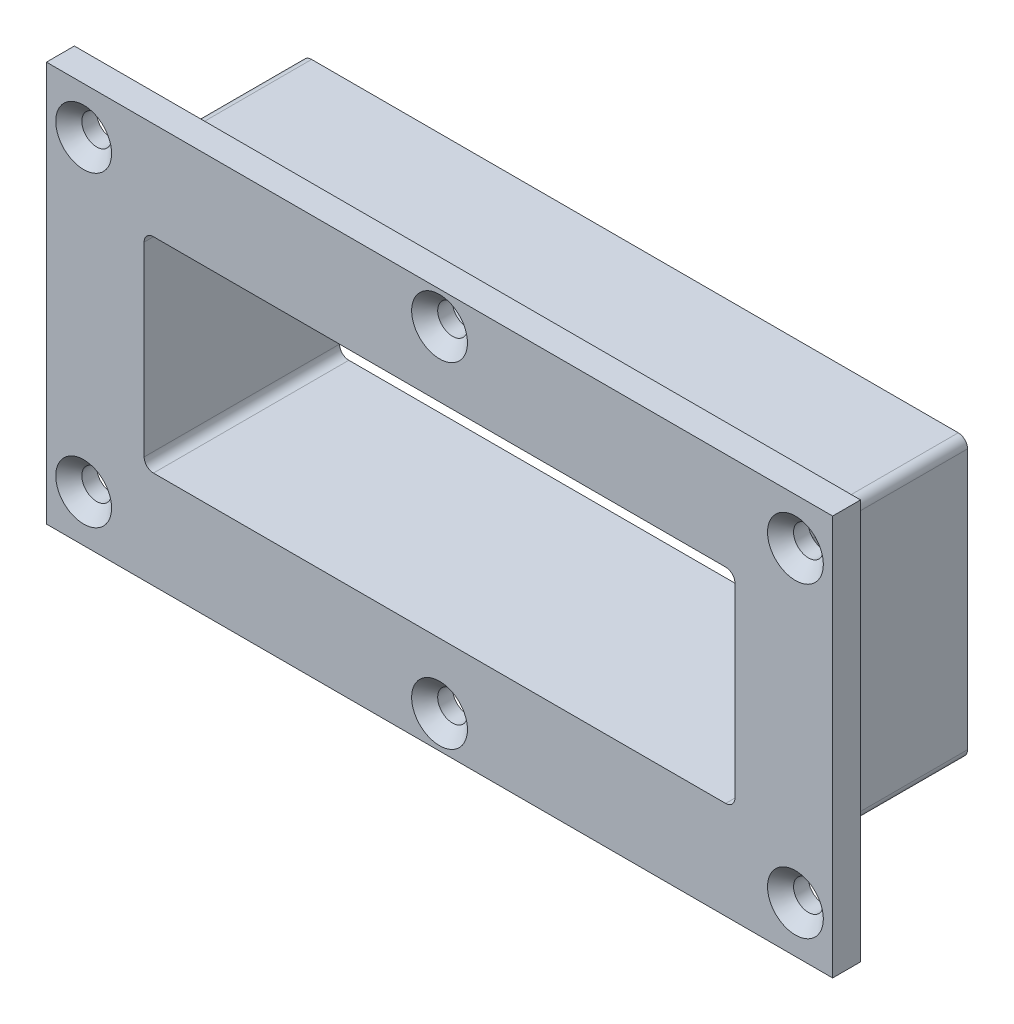
from build123d import *

# Parameters (mm, degrees)
SKETCH1_W                                         = 71.5
SKETCH1_H                                         = 30
SKETCH1_W_2                                       = 63.5
SKETCH1_H_2                                       = 22
BOSS_EXTRUDE1_DEPTH                               = 21
SKETCH2_W                                         = 71.5
SKETCH2_H                                         = 30
BOSS_EXTRUDE2_DEPTH                               = 3
SKETCH3_W                                         = 68.9
SKETCH3_H                                         = 27.4
SKETCH3_W_2                                       = 65.9
SKETCH3_H_2                                       = 24.4
CUT_EXTRUDE1_DEPTH                                = 1.5
SKETCH4_R                                         = 1.6
CUT_EXTRUDE2_DEPTH                                = 3
PILOT_HOLE_SIZE_PER_CROSS_FOR_HALF_CO_D           = 3.2
PILOT_HOLE_SIZE_PER_CROSS_FOR_HALF_CO_DEPTH       = 6.1
PILOT_HOLE_SIZE_PER_CROSS_FOR_HALF_CO_CSINK_D     = 6
PILOT_HOLE_SIZE_PER_CROSS_FOR_HALF_CO_CSINK_ANGLE = 90
PILOT_HOLE_SIZE_PER_CROSS_FOR_HALF_CO_TIP         = 0.96137699
FILLET1_R                                         = 1
FILLET2_R                                         = 1


with BuildPart() as part:
    # Sketch1 → Boss-Extrude1 (new body)
    with BuildSketch(Plane.XY):
        Rectangle(SKETCH1_W, SKETCH1_H)
        Rectangle(SKETCH1_W_2, SKETCH1_H_2, mode=Mode.SUBTRACT)
    extrude(amount=BOSS_EXTRUDE1_DEPTH)

    # Sketch2 → Boss-Extrude2 (add)
    with BuildSketch(Plane.XY.offset(21)):
        Polygon((42.25, 15), (42.25, -15), (42.25, -21.5), (-42.25, -21.5), (-42.25, -15), (-42.25, 15), (-42.25, 21.5), (42.25, 21.5), align=None)
        Rectangle(SKETCH2_W, SKETCH2_H, mode=Mode.SUBTRACT)
    extrude(amount=-BOSS_EXTRUDE2_DEPTH)

    # Sketch3 → Cut-Extrude1 (cut)
    with BuildSketch(Plane(origin=(0, 0, 0), x_dir=(-1, 0, 0), z_dir=(0, 0, -1))):
        Rectangle(SKETCH3_W, SKETCH3_H)
        Rectangle(SKETCH3_W_2, SKETCH3_H_2, mode=Mode.SUBTRACT)
    extrude(amount=-CUT_EXTRUDE1_DEPTH, mode=Mode.SUBTRACT)

    # Sketch4 → Cut-Extrude2 (cut)
    with BuildSketch(Plane(origin=(0, 0, 18), x_dir=(-1, 0, 0), z_dir=(0, 0, -1))):
        with Locations((-38.25, 16.5)):
            Circle(SKETCH4_R)
        with Locations((-38.25, -16.5)):
            Circle(SKETCH4_R)
        with Locations(Location((38.25, -16.5, 0), (0, 0, 180))):
            Circle(SKETCH4_R)
        with Locations(Location((38.25, 16.5, 0), (0, 0, 180))):
            Circle(SKETCH4_R)
        with Locations((0, -18)):
            Circle(SKETCH4_R)
        with Locations((0, 18)):
            Circle(SKETCH4_R)
    extrude(amount=-CUT_EXTRUDE2_DEPTH, mode=Mode.SUBTRACT)

    # Pilot hole size (% per cross) for half-countersunk wood screw, type 1
    with Locations(Plane.XY.offset(21)):
        with Locations((-38.25, 16.5), (-38.25, -16.5), (38.25, 16.5), (38.25, -16.5), (0, -18), (0, 18)):
            CounterSinkHole(PILOT_HOLE_SIZE_PER_CROSS_FOR_HALF_CO_D / 2, PILOT_HOLE_SIZE_PER_CROSS_FOR_HALF_CO_CSINK_D / 2, depth=PILOT_HOLE_SIZE_PER_CROSS_FOR_HALF_CO_DEPTH, counter_sink_angle=PILOT_HOLE_SIZE_PER_CROSS_FOR_HALF_CO_CSINK_ANGLE)
            with Locations((0, 0, -(PILOT_HOLE_SIZE_PER_CROSS_FOR_HALF_CO_DEPTH + PILOT_HOLE_SIZE_PER_CROSS_FOR_HALF_CO_TIP / 2))):  # 118° drill point
                Cone(0, PILOT_HOLE_SIZE_PER_CROSS_FOR_HALF_CO_D / 2, PILOT_HOLE_SIZE_PER_CROSS_FOR_HALF_CO_TIP, mode=Mode.SUBTRACT)

    # Fillet1
    fillet1_edges = [part.edges().sort_by_distance(p)[0] for p in [
        (-31.75, 11, 10.5),
        (-31.75, -11, 10.5),
        (31.75, -11, 10.5),
        (31.75, 11, 10.5),
        (34.45, 13.7, 0.75),
        (-34.45, 13.7, 0.75),
        (-34.45, -13.7, 0.75),
        (34.45, -13.7, 0.75),
        (32.95, -12.2, 0.75),
        (32.95, 12.2, 0.75),
        (-32.95, 12.2, 0.75),
        (-32.95, -12.2, 0.75),
    ]]
    fillet(fillet1_edges, radius=FILLET1_R)

    # Fillet2
    fillet2_edges = [part.edges().sort_by_distance(p)[0] for p in [
        (-35.75, -15, 9),
        (-35.75, 15, 9),
        (35.75, 15, 9),
        (35.75, -15, 9),
    ]]
    fillet(fillet2_edges, radius=FILLET2_R)


solid = part.part
